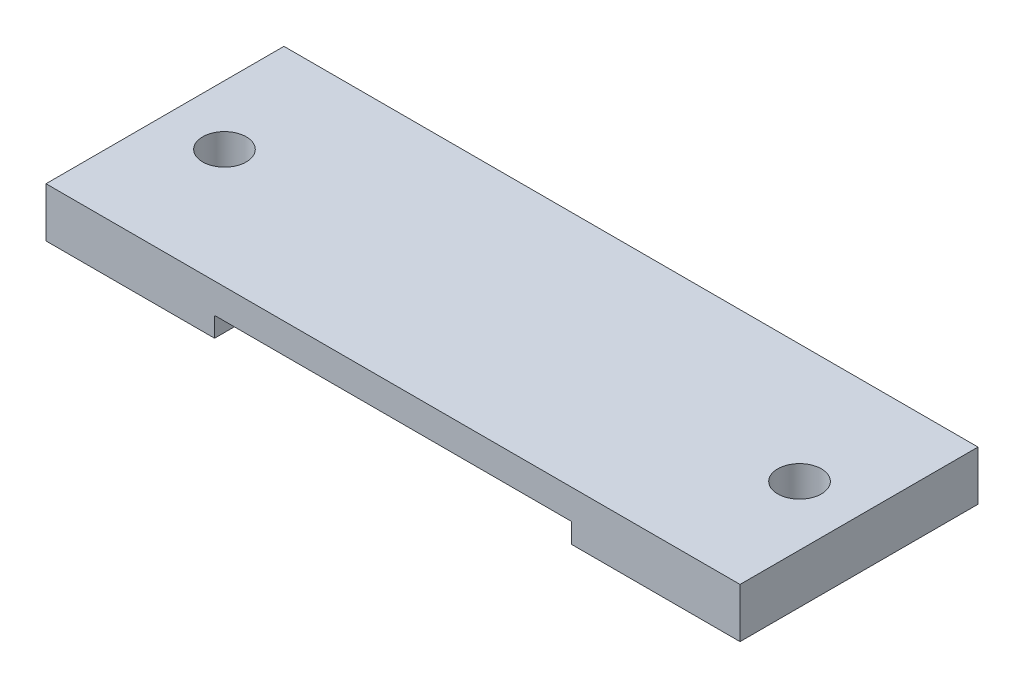
SolidWorks part; units mm, degrees
ref_plane "Front Plane" through (0, 0, 0) normal (0, 0, 1) x (1, 0, 0)
ref_plane "Top Plane" through (0, 0, 0) normal (0, 1, 0) x (1, 0, 0)
ref_plane "Right Plane" through (0, 0, 0) normal (1, 0, 0) x (0, 0, -1)
sketch "Sketch1" plane through (0, 0, 0) normal (0, 1, 0) x (1, 0, 0)
  line L1 (-175, 60) -> (175, 60)
  line L2 (-175, 60) -> (-175, -60)
  line L3 (-175, -60) -> (175, -60)
  line L4 (175, 60) -> (175, -60)
  line L5 (-175, 60) -> (175, -60) construction
  line L6 (-175, -60) -> (175, 60) construction
  point P0 (0, 0)
  dimension "D1" = 350
  dimension "D2" = 120
extrude "Boss-Extrude1" add sketch "Sketch1" along normal blind 25
sketch "Sketch2" plane through (0, 0, 60) normal (0, 0, 1) x (1, 0, 0)
  line L0 (-175, 0) -> (175, 0) construction
  line L1 (-90, -10) -> (90, -10)
  line L2 (-90, -10) -> (-90, 10)
  line L3 (-90, 10) -> (90, 10)
  line L4 (90, -10) -> (90, 10)
  line L5 (-90, -10) -> (90, 10) construction
  line L6 (-90, 10) -> (90, -10) construction
  point P0 (0, 0)
  dimension "D1" = 180
  dimension "D2" = 10
extrude "Cut-Extrude1" cut sketch "Sketch2" against normal through all
sketch "Sketch3" plane through (0, 25, 0) normal (0, 1, 0) x (1, 0, 0)
  line L0 (0, 0) -> (0, 81.398) construction
  circle A0 centre (-145, 0) radius 11
  circle A1 centre (145, 0) radius 11
  dimension "D1" = 22
  dimension "D2" = 290
extrude "Cut-Extrude2" cut sketch "Sketch3" against normal blind 25
fillet "Fillet1" radius 0.5 2 edges at (90, 10, 0) (-90, 10, 0)
